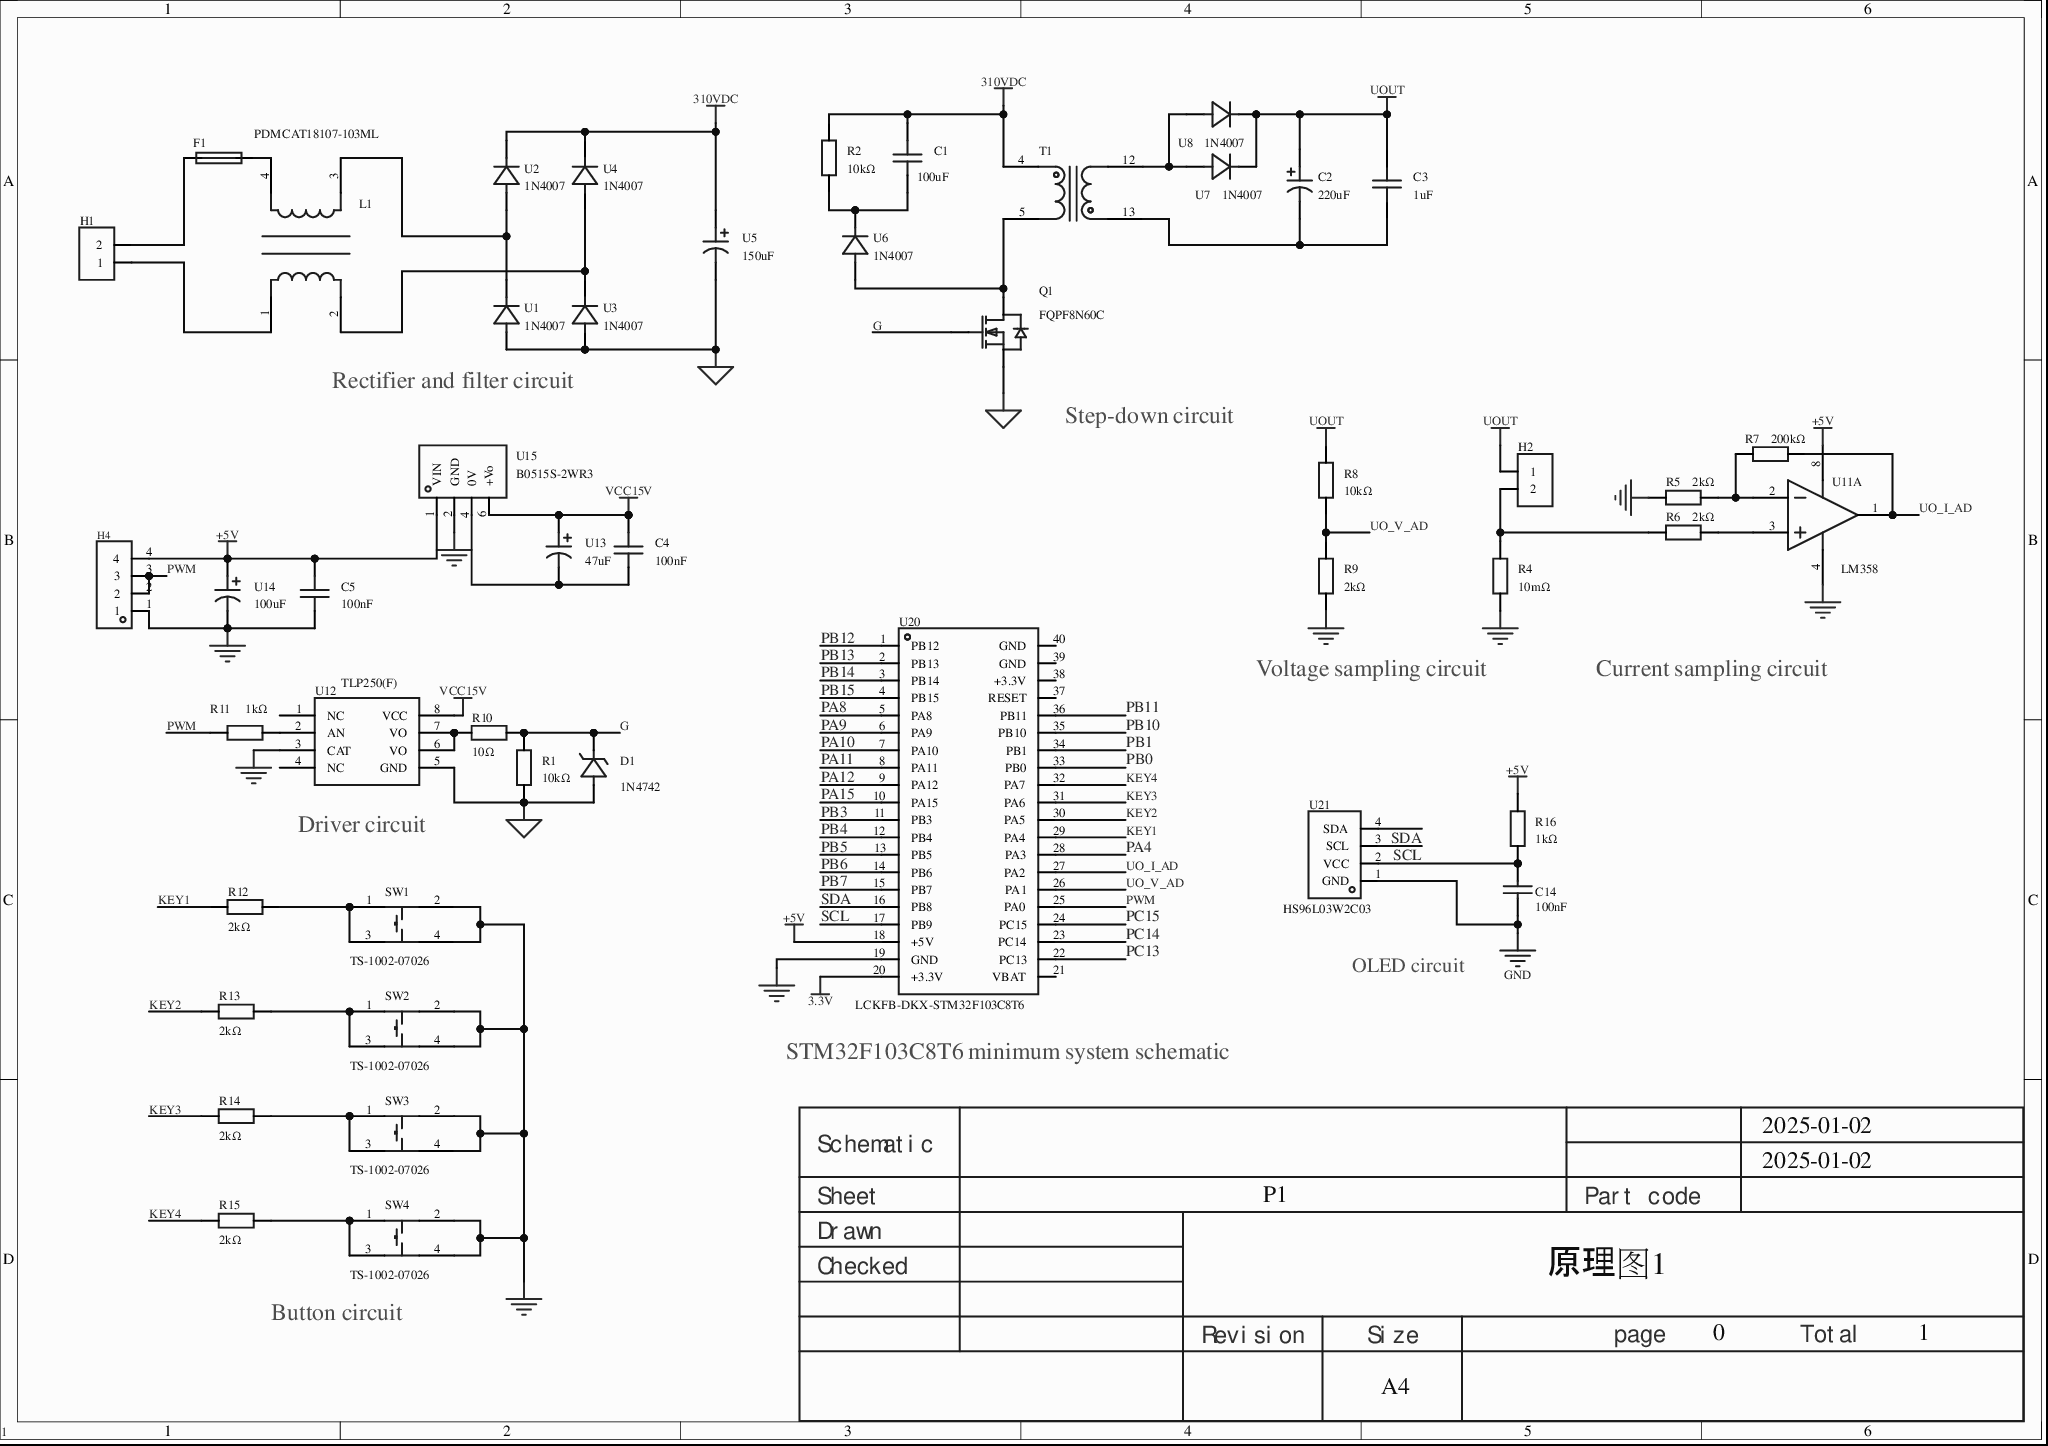
[diagram p0: MISC75075-3.schdoc]
# Altium project MISC75075-2.PrjPcb
1 sheet, 48 parts. Net scope: global (net labels, ports and power ports of the same name join across sheets).
Board file: MISC75075.pcbdoc

## Sheet MISC75075-3.schdoc
size 297 x 209 mm; Version: V1.0; @Project Name: MISC75075; @Page Count: 1; @Update Date: 2025-01-02; @Create Date: 2025-01-02; @Schematic Name: MISC75075; @Page No: 0; @Board Name: MISC75075; @Create Time: 18:15:10; @Update Time: 23:09:33

### Parts
C1  100uF  [CAP-TH_L12.0-W5.5-P10.00-D1.0]
C2  220uF  [CAP-TH_BD8.0-P3.50-D0.6-FD]
C3  1uF  [CAP-TH_L5.8-W3.6-P5.0-D0.6]
C4  100nF  [CAP-TH_L5.0-W2.5-P5.00-D1.0]
C5  100nF  [CAP-TH_L5.0-W2.5-P5.00-D1.0]
C14  100nF  [C0805]
D1  1N4742  [DO-41_BD2.4-L4.7-P8.70-D0.8-FD]
F1  5F.2000210000R1  [FUSE-SMD_5-20MM]  (value not drawn)
H1  (no value)  [HDR-TH_2P-P2.54-V-F]
H2  (no value)  [HDR-TH_2P-P2.54-V-F]
H4  (no value)  [HDR-TH_4P-P2.54-V-F]
L1  PDMCAT18107-103ML  [IND-TH_4P-L22.0-W12.0-TR]
Q1  FQPF8N60C  [TO-220F-3_L10.2-W4.9-P2.54-L]
R1  10kΩ  [Res_1/4W]
R2  10kΩ  [Res_1W]
R4  10mΩ  [Res_1/4W]
R5  2kΩ  [Res_1/4W]
R6  2kΩ  [Res_1/4W]
R7  200kΩ  [Res_1/4W]
R8  10kΩ  [Res_1/4W]
R9  2kΩ  [Res_1/4W]
R10  10Ω  [Res_1/4W]
R11  1kΩ  [Res_1/4W]
R12  2kΩ  [Res_1/4W]
R13  2kΩ  [Res_1/4W]
R14  2kΩ  [Res_1/4W]
R15  2kΩ  [Res_1/4W]
R16  1kΩ  [Res_1/4W]
SW1  TS-1002-07026  [SW-TH_4P-L6.0-W6.0-P4.50-LS6.5]
SW2  TS-1002-07026  [SW-TH_4P-L6.0-W6.0-P4.50-LS6.5]
SW3  TS-1002-07026  [SW-TH_4P-L6.0-W6.0-P4.50-LS6.5]
SW4  TS-1002-07026  [SW-TH_4P-L6.0-W6.0-P4.50-LS6.5]
T1  (no value)  [dip2_8_5mm_35MM]
U1  1N4007  [DO-41_BD2.4-L4.7-P8.70-D0.6-RD]
U2  1N4007  [DO-41_BD2.4-L4.7-P8.70-D0.6-RD]
U3  1N4007  [DO-41_BD2.4-L4.7-P8.70-D0.6-RD]
U4  1N4007  [DO-41_BD2.4-L4.7-P8.70-D0.6-RD]
U5  150uF  [CAP-TH_BD18.0-P7.50-D0.8-FD]
U6  1N4007  [DO-41_BD2.4-L4.7-P8.70-D0.6-RD]
U7  1N4007  [DO-41_BD2.4-L4.7-P8.70-D0.6-RD]
U8  1N4007  [DO-41_BD2.4-L4.7-P8.70-D0.6-RD]
U11  LM358  [DIP-8_L9.8-W6.4-P2.54-LS7.6-BL]  (part A of 2)
U12  TLP250(F)  [DIP-8_L9.4-W6.4-P2.54-LS9.1-BL]
U13  47uF  [CAP-TH_BD5.0-P2.00-D0.5-FD]
U14  100uF  [CAP-TH_BD5.0-P2.00-D0.5-FD]
U15  B0515S-2WR3  [SIP-4_L19.5-W7.0-P2.54-L]
U20  LCKFB-DKX-STM32F103C8T6  [CONN-TH_L53.3-W22.9_STM32F103C8T6-CARD]
U21  HS96L03W2C03  [OLED-TH_L27.8-W27.2-P2.54_C9900033791]

### Nets
3.3V: U20.20(+3.3V)
310VDC: C1.2 R2.2 T1.4 U2.1(C) U4.1(C) U5.1
+5V: C5.1 H4.4 R16.2 U11.8(VCC) U14.1 U15.1(VIN) U20.18(+5V)
AGND: D1.1(A) Q1.3(S) R1.2 U1.2(A) U3.2(A) U5.2 U12.5(GND)
GND: C5.2 C14.1 H4.1 R4.1 R5.1 R9.1 SW1.2 SW1.4 SW2.2 SW2.4 SW3.2 SW3.4 SW4.2 SW4.4 U11.4(GND) U12.3(CAT) U14.2 U15.2(GND) U20.19(GND) U21.1(GND)
UOUT: C2.1 C3.2 H2.1 R8.2 U7.1(C) U8.1(C)
VCC15V: C4.1 U12.8(VCC) U13.1 U15.6(+Vo)
G: D1.2(K) Q1.1(G) R1.1 R10.2
KEY1: R12.2 U20.29(PA4)
KEY2: R13.2 U20.30(PA5)
KEY3: R14.2 U20.31(PA6)
KEY4: R15.2 U20.32(PA7)
PA4: U20.28(PA3)
PA8: U20.5(PA8)
PA9: U20.6(PA9)
PA10: U20.7(PA10)
PA11: U20.8(PA11)
PA12: U20.9(PA12)
PA15: U20.10(PA15)
PB0: U20.33(PB0)
PB1: U20.34(PB1)
PB3: U20.11(PB3)
PB4: U20.12(PB4)
PB5: U20.13(PB5)
PB6: U20.14(PB6)
PB7: U20.15(PB7)
PB10: U20.35(PB10)
PB11: U20.36(PB11)
PB12: U20.1(PB12)
PB13: U20.2(PB13)
PB14: U20.3(PB14)
PB15: U20.4(PB15)
PC13: U20.22(PC13)
PC14: U20.23(PC14)
PC15: U20.24(PC15)
PWM: H4.2 H4.3 R11.1 U20.25(PA0)
SCL: U20.17(PB9) U21.3(SCL)
SDA: U20.16(PB8) U21.4(SDA)
UO_I_AD: R7.2 U11.1(OUT1) U20.27(PA2)
UO_V_AD: R8.1 R9.2 U20.26(PA1)
NetC1_1: C1.1 R2.1 U6.1(C)
NetC2_2: C2.2 C3.1 T1.13
NetC4_2: C4.2 U13.2 U15.4(0V)
NetC14_2: C14.2 R16.1 U21.2(VCC)
NetF1_1: F1.1 H1.2
NetF1_2: F1.2 L1.4
NetH1_1: H1.1 L1.1
NetH2_2: H2.2 R4.2 R6.1
NetL1_2: L1.2 U3.1(C) U4.2(A)
NetL1_3: L1.3 U1.1(C) U2.2(A)
NetQ1_2: Q1.2(D) T1.5 U6.2(A)
NetR5_2: R5.2 R7.1 U11.2(IN1-)
NetR6_2: R6.2 U11.3(IN1+)
NetR10_1: R10.1 U12.6(VO) U12.7(VO)
NetR11_2: R11.2 U12.2(AN)
NetR12_1: R12.1 SW1.1 SW1.3
NetR13_1: R13.1 SW2.1 SW2.3
NetR14_1: R14.1 SW3.1 SW3.3
NetR15_1: R15.1 SW4.1 SW4.3
NetT1_12: T1.12 U7.2(A) U8.2(A)

Not connected (* = marked no-connect by the designer): U12 1(NC)* 4(NC)*; U20 21(VBAT) 37(RESET) 38(+3.3V) 39(GND) 40(GND)

### Notes on the sheet
- Rectifier and filter circuit
- Step-down circuit
- Voltage sampling circuit
- Current sampling circuit
- Driver circuit
- OLED circuit
- (near U20) STM32F103C8T6 minimum system schematic
- (near SW4) Button circuit
- 2025-01-02
- Schematic
- Sheet
- P1
- Part code
- Checked
- Drawn
- 原理图1
- Revision
- Size
- A4
- page
- 0
- Total
- 1

### Library data of the parts
C1 = KP104J2J1006: Capacitance:100nF;Tolerance:±5%;Rated voltage:630V;Operating temperature:-40℃~+100℃;; Manufacturer: KYET(科雅); AddInBom: yes; ModelId: af4d87f22de946f3b87e9bc308909498; ModelName: CAP-TH_L12.0-W5.5-H10.0-P10.0; ModelTransform: 472.44,216.535,0,0,0,0,0,0,-137.795; Tolerance: ±5%; Voltage Rated: 630V; Symbol: KP104J2J1006; Value: 100uF; Device: KP104J2J1006; LCSC Part Name: 100nF ±5% 630V; ManufacturerPart: KP104J2J1006; Supplier Footprint: 插件,P=10mm; JLCPCB Part Class: Extended library; Datasheet: https://atta.szlcsc.com/upload/public/pdf/source/20190521/C390130_D3C9634A93402282F0F48D613188513C.pdf; Supplier: LCSC; ConvertToPcb: yes; FootprintName: CAP-TH_L12.0-W5.5-P10.00-D1.0; Operating Temperature: -40℃~+100℃
C2 = 01EC3470: Capacitance:220uF;Tolerance:±20%;Rated voltage:50V;Ripple current:350mA@120kHz;ESR:-;; Manufacturer: KNSCHA(科尼盛); AddInBom: yes; ModelId: a2c936ec27754f809f3966430e36f767; ModelName: CAP-TH_D8.0-H8.0-P3.50; ModelTransform: 314.96,314.862,0,180,0,0,0,0,-137.795; Tolerance: ±20%; Rated Voltage: 50V; φD: 8mm; L: 12mm; Lifetime @ Temp: 2000hrs@105℃; Symbol: 01EC3470; Device: 01EC3470; LCSC Part Name: 220uF ±20% 50V; SupplierPart: C2836445; ManufacturerPart: 01EC3470; Supplier Footprint: 插件,D8xL12mm; JLCPCB Part Class: Extended library; Datasheet: https://atta.szlcsc.com/upload/public/pdf/source/20210528/C2836445_4EB3DEC3C45633977FB5495C9B2E1697.pdf; Supplier: LCSC; ConvertToPcb: yes; FootprintName: CAP-TH_BD8.0-P3.50-D0.6-FD; Value: 220uF; Ripple Current: 350mA@120kHz; Equivalent Series Resistance(ESR): -; Lead Spacing: 3.5mm; Operating Temperature: -40℃~+105℃
C3 = 178MU0005: Capacitance:1uF;Tolerance:±10%;Rated voltage:50V;Temperature coefficient:X7R;; Manufacturer: KNSCHA(科尼盛); AddInBom: yes; ModelId: 67fba78a874e4dacbebdaf4238731352; ModelTransform: 228.346,142.1257,0,0,0,0,0,0,-196.85; Tolerance: ±10%; Voltage Rated: 50V; Temperature Coefficient: X7R; Symbol: 178MU0005; Device: 178MU0005; LCSC Part Name: 1uF ±10% 50V; SupplierPart: C5632429; ManufacturerPart: 178MU0005; Supplier Footprint: 插件,P=5.08mm; JLCPCB Part Class: Extended library; Datasheet: https://atta.szlcsc.com/upload/public/pdf/source/20230506/91591964510408E842F19503EB051561.pdf; Supplier: LCSC; ConvertToPcb: yes; FootprintName: CAP-TH_L5.8-W3.6-P5.0-D0.6; ModelName: CAP-TH_L5.8-W3.6-P5.0-D0.6; Value: 1uF
C4 C5 = CC1H104MC1FD3F6C10MF: Capacitance:100nF;Tolerance:±20%;Rated voltage:50V;Temperature coefficient:Y5V;; Manufacturer: Dersonic(德尔创); AddInBom: yes; ModelId: 08e3d7481fc7486bb1b263873f51e1e1; ModelName: CAP-TH_BD5.0-W2.5-P5.08; ModelTransform: 224.652,98.425,0,0,0,0,-0.005,0,-137.795; Tolerance: ±20%; Voltage Rated: 50V; Temperature Coefficient: Y5V; φD: 6mm; Body Thickness: 2.2mm; Symbol: CC1H104MC1FD3F6C10MF; Device: CC1H104MC1FD3F6C10MF; Supplier: LCSC; Supplier Part: C254085; Manufacturer Part: CC1H104MC1FD3F6C10MF; Value: 100nF; JLCPCB Part Class: Extended library; LCSC Part Name: 100nF ±20% 50V; Supplier Footprint: 插件,P=5.08mm; Datasheet: https://atta.szlcsc.com/upload/public/pdf/source/20200826/C254085_159DD65BF32BF11C9168D341BCE23E6F.pdf; ConvertToPcb: yes; FootprintName: CAP-TH_L5.0-W2.5-P5.00-D1.0; Lead Spacing: 5.08mm
C14 = CC0805KRX7R9BB104: Manufacturer: YAGEO; Convert to PCB: yes; Origin Footprint: C0805; Device: CC0805KRX7R9BB104; Symbol: 100nF; Add into BOM: yes; Supplier: LCSC; ManufacturerPart: CC0805KRX7R9BB104; SupplierPart: C49678; JLCPCB Part Class: Basic; FootprintName: C0805
D1 = 1N4742: Diode configuration:Single;Zener voltage (nominal):12V;Zener voltage (range):11.45V~12.95V;Power:1W;Tolerance:±5%;; Manufacturer: LGE(鲁光); AddInBom: yes; ModelId: 6de1e9b71a0d4751b4e9df530304c1a3; ModelName: DO-41_D2.4-L4.7-P8.70; ModelTransform: 374.015,94.428,0,180,0,0,0,0,-137.795; Diode Configuration: Single; Zener Voltage (Nom): 12V; Reverse Leakage Current (Ir): 3uA; Power Dissipation: 1W; Zener Impedance (Zzt): 9Ω; Tolerance: ±5%; Symbol: 1N4742; Device: 1N4742; Supplier: LCSC; Supplier Part: C5174492; Manufacturer Part: 1N4742; JLCPCB Part Class: Extended library; LCSC Part Name: 1N4742; Supplier Footprint: DO-41; Datasheet: https://atta.szlcsc.com/upload/public/pdf/source/20220915/859F92BB52C22EFA9D12B90684DCEAFE.pdf; ConvertToPcb: yes; FootprintName: DO-41_BD2.4-L4.7-P8.70-D0.8-FD; Zener Voltage (Range): 11.45V~12.95V
F1 = 5F.2000210000R1: Type:glass tube fuse;Rated current:2A;; Manufacturer: xcfuse(旭程); Symbol: 2A 250VACGlass tube fuse; AddInBom: yes; ModelId: 9c1981df6d6347b8ba6f449df7014a94; ModelName: FUSE-SMD_D5.0-L20.0; ModelTransform: 787.4,204.724,0,0,0,0,0,0,0; Current Rating: 2A; Device: 5F.2000210000R1; LCSC Part Name: 玻璃管保险丝; SupplierPart: C3117; ManufacturerPart: 5F.2000210000R1; Supplier Footprint: D5.2xL20mm; JLCPCB Part Class: Extended library; Datasheet: https://atta.szlcsc.com/upload/public/pdf/source/20180404/C3117_7632A939106813D02D9AA950EAD91ADA.pdf; Supplier: LCSC; ConvertToPcb: yes; FootprintName: FUSE-SMD_5-20MM; Type: Glass tube fuse
H1 H2 = HDR-F_2.54_1x2P: Manufacturer: BOOMELE(博穆精密); Manufacturer Part: 2.54-1*2P母; Symbol: Header-Female-2.54_1x2; ConvertToPcb: yes; ModelId: a9450ef445564560a104363b9aacde4e; ModelName: HDR-TH_2P-P2.54-F-LI-1X2P; ModelTransform: 215.7476,98.425,0,0,0,0,0,0,-129.921; Supplier Part: C49661; Device: HDR-F_2.54_1x2P; Supplier: LCSC; JLCPCB Part Class: Extended Part; AddInBom: yes; Supplier Footprint: 插件; FootprintName: HDR-TH_2P-P2.54-V-F
H4 = HDR-F_2.54_1x4P: Manufacturer: BOOMELE(博穆精密); Manufacturer Part: 2.54-1*4P母; Symbol: 2.54-1*4P female; ConvertToPcb: yes; ModelId: 57daaad411c24bd7bd5d06edf5c4d16b; ModelName: HDR-TH_4P-P2.54-F-LI-1X4P; ModelTransform: 415.7472,98.425,0,0,0,0,0,0,-118.11; Device: HDR-F_2.54_1x4P; Supplier: LCSC; Supplier Part: C2718488; JLCPCB Part Class: Extended Part; AddInBom: yes; Supplier Footprint: 插件; FootprintName: HDR-TH_4P-P2.54-V-F
L1 = PDMCAT18107-103ML: Lines:2;Inductance @ frequency:10mH@1kHz;DC resistance (DCR):55mΩ;; Manufacturer: PROD(谱罗德); AddInBom: yes; ModelId: 33e9bcd339054a48809664c675272bbc; ModelTransform: 897.784,474.64948,0,0,0,0,0,0,-196.85; Number of Lines: 2; Withstanding Voltage: 600V@AC,3secs; Current Rating: 3A; Voltage Rating - DC: 600V; Voltage Rating: 600VAC; DC Resistance (DCR): 55mΩ; Symbol: PDMCAT18107-103ML; Device: PDMCAT18107-103ML; LCSC Part Name: 两路 插件共模滤波器; SupplierPart: C2832691; ManufacturerPart: PDMCAT18107-103ML; Supplier Footprint: 插件,22x12mm; JLCPCB Part Class: Extended library; Datasheet: https://atta.szlcsc.com/upload/public/pdf/source/20210602/C2832691_EACDFDD6E373F5FB74BA58CC338ECD64.pdf; Supplier: LCSC; ConvertToPcb: yes; FootprintName: IND-TH_4P-L22.0-W12.0-TR; ModelName: IND-TH_4P-L22.0-W12.0-TR; Inductance @ Frequency: 10mH@1kHz; Operating Temperature: -25℃~+85℃
Q1 = FQPF8N60C: Type:1 N-channel;Drain-source voltage (Vdss):600V;Continuous drain current (Id):7.5A;On-resistance (RDS(on)@Vgs,Id):1.2Ω@10V,3.75A;Power (Pd):48W;Gate threshold voltage (Vgs(th)@Id):4V@250uA;; Manufacturer: onsemi(安森美); AddInBom: yes; ModelId: 9569686711e34fe2ae87dea58cf6ecc7; ModelName: ITO-220AB_3PIN-L10.5-W5.0-H20.0-P2.54; ModelTransform: 405.511,185.039,0,0,0,0,0,29.524,-393.701; Drain Source Voltage (Vdss): 600V; Continuous Drain Current (Id): 7.5A; Power Dissipation (Pd): 48W; Total Gate Charge (Qg@Vgs): 36nC@10V; Input Capacitance (Ciss@Vds): 1.255nF@25V; Symbol: FQPF8N60C; Device: FQPF8N60C; LCSC Part Name: 1个N沟道 耐压:600V 电流:7.5A; SupplierPart: C2703; ManufacturerPart: FQPF8N60C; Supplier Footprint: TO-220F-3; JLCPCB Part Class: Extended library; Datasheet: https://atta.szlcsc.com/upload/public/pdf/source/20120409/1457706467535.pdf; Supplier: LCSC; ConvertToPcb: yes; FootprintName: TO-220F-3_L10.2-W4.9-P2.54-L; Type: 1 N-channel; Drain Source On Resistance (RDS(on)@Vgs,Id): 1.2Ω@10V,3.75A; Gate Threshold Voltage (Vgs(th)@Id): 4V@250uA; Operating Temperature: -55℃~+150℃@(Tj)
R1 R4-R16 = Res_AXIAL-1/4W: Symbol: Resistor; AddInBom: yes; ModelId: 463263665006444ab7a47bd11b0cf956; ModelName: RES-TH_BD2.4-L6.3-P10.30-D0.6; ModelTransform: 427.165,94.32816,0,0,0,0,0,0,-196.85; Device: Res_AXIAL-1/4W; Supplier Footprint: 轴向引线; ConvertToPcb: yes; FootprintName: Res_1/4W
  R1 R8: Value: 10kΩ
  R4: Value: 10mΩ
  R5 R6 R9 R12-R15: Value: 2kΩ
  R7: Value: 200kΩ
  R10: Value: 10Ω
  R11 R16: Value: 1kΩ
R2 = Res_AXIAL-1W: Symbol: Resistor; ConvertToPcb: yes; ModelId: f1f7cfb3d56f4763951150e77c261d09; ModelName: RES-TH_BD4.5-L11.5-P15.50-D0.8; ModelTransform: 641.71,177.16,374,0,0,0,0,0,-190; Device: Res_AXIAL-1W; AddInBom: yes; Supplier Footprint: 轴向引线; Value: 10kΩ; FootprintName: Res_1W
SW1-SW4 = TS-1002-07026: Circuit structure:Single-pole single-throw;Button shape:Round button;Mounting style:Through-hole;Switch length:6mm;Switch width:6mm;Switch height:7mm;Contact current:50mA;Rated voltage (DC):12V;With LED:-;Mechanical life:-;; Manufacturer: XUNPU(讯普); AddInBom: yes; ModelId: 20eee248bc684ccd8cbdbb1d0d91ec6f; ModelName: SW-TH_4P-L6.0-W6.0-H5.0-LS6.5-P4.50; ModelTransform: 236.22,323.03,0,90,0,0,0,0,-137.795; Switch Length: 6mm; Switch Height: 7mm; Contact Current: 50mA; Voltage Rating (DC): 12V; Symbol: TS-1002-07026; Device: TS-1002-07026; LCSC Part Name: 6*6*7mm 直插 轻触开关; SupplierPart: C455095; ManufacturerPart: TS-1002-07026; Supplier Footprint: 插件,6x6mm; JLCPCB Part Class: Extended library; Datasheet: https://atta.szlcsc.com/upload/public/pdf/source/20231108/52BC6409AB52B6746CCC051A15664904.pdf; Supplier: LCSC; ConvertToPcb: yes; FootprintName: SW-TH_4P-L6.0-W6.0-P4.50-LS6.5; Circuit: Single-pole single-throw; Actuator Style: Round button; Mounting Style: Through-hole; Switch Width: 6mm; With Lamp: -; Mechanical Life: -
T1 = T220Vto18V: Primary voltage:-;Secondary voltage:-;Output current:-;Power:2W;; AddInBom: yes; Power: 2W; Primary Winding: Dual; Isolation Voltage: 3kV; Device: T220Vto18V; LCSC Part Name: 小体积隔离变压器; ConvertToPcb: yes; Primary Side Voltage: -; Secondary Side Voltage: -; Output Current: -; Secondary Winding: Dual; SymbolName: T220Vto18V; FootprintName: dip2_8_5mm_35MM
U1-U4 U6-U8 = 1N4007_C5261026: Manufacturer: CJ(江苏长电/长晶); AddInBom: yes; ModelId: 6de1e9b71a0d4751b4e9df530304c1a3; ModelName: DO-41_D2.4-L4.7-P8.70; ModelTransform: 374.015,94.428,0,0,0,0,0,0,-137.795; Symbol: 1N4007_C5261026; Device: 1N4007_C5261026; LCSC Part Name: 1N4007; SupplierPart: C5261026; ManufacturerPart: 1N4007; Supplier Footprint: DO-41; JLCPCB Part Class: Extended library; Datasheet: https://atta.szlcsc.com/upload/public/pdf/source/20221115/D7EC334A50D1A4CD81D868035690309F.pdf; Supplier: LCSC; ConvertToPcb: yes; FootprintName: DO-41_BD2.4-L4.7-P8.70-D0.6-RD
U5 = CD1101572GM1836VFL: Capacitance:150uF;Rated voltage:400V;; Manufacturer: HRK(鸿瑞凯电子); AddInBom: yes; ModelId: 050876a6b8f84a9faf6465d78b360231; ModelName: CAP-TH_BD18.0-H30.0-P7.5; ModelTransform: 709.0537,708.516,0,0,0,0,0,0,-137.795; Rated Voltage: 400V; Symbol: CD1101572GM1836VFL; Device: CD1101572GM1836VFL; LCSC Part Name: 150uF 400V; SupplierPart: C7493882; ManufacturerPart: CD1101572GM1836VFL; Supplier Footprint: 插件,D18xL36mm; JLCPCB Part Class: Extended library; Supplier: LCSC; ConvertToPcb: yes; FootprintName: CAP-TH_BD18.0-P7.50-D0.8-FD; Value: 150uF
U11 = LM358_C5157924: Manufacturer: Gcore(扬州国芯); Relevance: []; AddInBom: yes; ModelId: ab479eee877a4d169ad0de4d5fd28296; ModelTransform: 385.826,309.842,0,0,0,0,0,0,-137.795; Symbol: LM358_C5157924; Device: LM358_C5157924; LCSC Part Name: LM358; SupplierPart: C5157924; ManufacturerPart: LM358; Supplier Footprint: DIP-8; JLCPCB Part Class: Extended library; Datasheet: https://atta.szlcsc.com/upload/public/pdf/source/20220906/3ACE6D6B047AB904F15AF865A5390D58.pdf; Supplier: LCSC; ConvertToPcb: yes; FootprintName: DIP-8_L9.8-W6.4-P2.54-LS7.6-BL; ModelName: DIP-8_L9.8-W6.4-P2.54-LS7.6-BL
U12 = TLP250(F): Input type:DC;Supply voltage:10V~35V;Common-mode transient immunity CMTI:5kV/us;Propagation delay tpLH/tpHL:500ns;500ns;; Manufacturer: TOSHIBA(东芝); AddInBom: yes; ModelId: 5746b540d01a4d1b9eb6b4f989297bc7; ModelName: DIP-8_L9.8-W6.6-H3.5-LS7.62-P2.54; ModelTransform: 385.826,311.8104,0,0,0,0,0,-0.0005,-118.11; Input Type: DC; Isolation Voltage(rms): 2.5kV; Common Mode Transient Immunity (CMTI): 5kV/us; Number of Channels: 1; Symbol: TLP250(F); Device: TLP250(F); Supplier: LCSC; Manufacturer Part: TLP250(F); Supplier Part: C4078; JLCPCB Part Class: Extended library; LCSC Part Name: DC输入 1通道 隔离电压(rms):2500V; Supplier Footprint: DIP-8; Datasheet: https://atta.szlcsc.com/upload/public/pdf/source/20210413/C2802426_0116EA7D297E93B6CB771644BB38F5D7.pdf; ConvertToPcb: yes; FootprintName: DIP-8_L9.4-W6.4-P2.54-LS9.1-BL; Supply Voltage: 10V~35V; Propagation Delay tpLH/tpHL: 500ns; 500ns; Operating Temperature: -20℃~+85℃
U13 U14 = KM1E470M0507: Capacitance:47uF;Tolerance:±20%;Rated voltage:25V;Ripple current:80mA@120kHz;ESR:-;; Manufacturer: ROQANG(容强); AddInBom: yes; ModelId: aba3b94bdab6406eb4f45c9c765c730e; ModelTransform: 196.85,196.517,0,0,0,0,0,0,-196.85; Tolerance: ±20%; Rated Voltage: 25V; φD: 5mm; L: 7mm; Lifetime @ Temp: 2000hrs@105℃; Symbol: KM1E470M0507; Device: KM1E470M0507; LCSC Part Name: 47uF ±20% 25V; ManufacturerPart: KM1E470M0507; Supplier Footprint: 插件,D5xL7mm; JLCPCB Part Class: Extended library; Datasheet: https://atta.szlcsc.com/upload/public/pdf/source/20210825/43CC5C3A3C9845108B639C21E16A1224.pdf; Supplier: LCSC; ConvertToPcb: yes; FootprintName: CAP-TH_BD5.0-P2.00-D0.5-FD; ModelName: CAP-TH_BD5.0-P2.00-D0.5-FD; Ripple Current: 80mA@120kHz; Equivalent Series Resistance(ESR): -; Lead Spacing: 2mm; Operating Temperature: -40℃~+105℃
  U13: SupplierPart: C2874001; Value: 47uF
  U14: Value: 100uF
U15 = B1215S-2WR3_C5369480: 100% domestically produced. B1215S-2WR3 is designed for board-level power systems that need an isolated voltage separate from the input supply. Suitable for: 1) input supply with stable voltage (voltage variation ±10%Vin); 2) input-output isolation required (isolation voltage ≤1500VDC); 3) low output voltage stability requirement; 4) typical applications: pure digital circuits, general low-frequency analog circuits, relay drive circuits, data exchange circuits. Features: fixed voltage input, isolated unregulated output, 2W, isolation voltage: 1500VDC, efficiency: up to 84%,; Manufacturer: YLPTEC(易川); AddInBom: yes; ModelId: 14e9d63c0e5a4a2bb8494eb97d019878; ModelTransform: 771.652,275.59,0,0,0,0,53.15,-101.654,-196.85; Manufacturer Part: B0515S-2WR3; Symbol: B1215S-2WR3_C5369480; Device: B1215S-2WR3_C5369480; LCSC Part Name: DC-DC 输入电压10.8V~13.2V 输出电压15V输出功率2W133mA; SupplierPart: C5369480; Supplier Footprint: SIP-4; JLCPCB Part Class: Extended library; Datasheet: https://atta.szlcsc.com/upload/public/pdf/source/20230427/82014D73CB8555D1D44C1887F1D9A3CE.pdf; Supplier: LCSC; ConvertToPcb: yes; FootprintName: SIP-4_L19.5-W7.0-P2.54-L; ModelName: SIP-4_L19.5-W7.0-P2.54-L
U20 = LCKFB-DKX-STM32F103C8T6: Manufacturer: 立创开发板; AddInBom: yes; Symbol: LCKFB-DKX-STM32F103C8T6; Device: LCKFB-DKX-STM32F103C8T6; LCSC Part Name: 立创·地阔星-STM32F103C8T6开发板; SupplierPart: C22396880; ManufacturerPart: LCKFB-DKX-STM32F103C8T6; Supplier Footprint: -; JLCPCB Part Class: Extended library; Datasheet: https://atta.szlcsc.com/upload/public/pdf/source/20240801/7EEF69F7480DF7C6DA98696664D658D4.pdf; Supplier: LCSC; ConvertToPcb: yes; FootprintName: CONN-TH_L53.3-W22.9_STM32F103C8T6-CARD
U21 = HS96L03W2C03: Main controller chip:SSD1315;Interface type:I2C;Size (inch):0.96;Pixel resolution:128x64;; Manufacturer: HS(汉昇); AddInBom: yes; ModelId: bb65183306db4ca69fb52250be49b00e; ModelTransform: 1070.864,1094.486,0,0,0,0,0,-468.503,0; Interface Type: I2C; Pixel Resolution: 128x64; Symbol: HS96L03W2C03; Device: HS96L03W2C03; LCSC Part Name: 0.96寸OLED显示屏窄白光IIC; SupplierPart: C5248080; ManufacturerPart: HS96L03W2C03; Supplier Footprint: -; JLCPCB Part Class: Extended library; Datasheet: https://atta.szlcsc.com/upload/public/pdf/source/20230627/763D01F79A90007632F098068C7C8AD9.pdf; Supplier: LCSC; ConvertToPcb: yes; FootprintName: OLED-TH_L27.8-W27.2-P2.54_C9900033791; ModelName: OLED-TH_L27.8-W27.2-P2.54_C9900033791; Main Control Chip: SSD1315; Size: 0.96; Operating Temperature: -40℃~+70℃